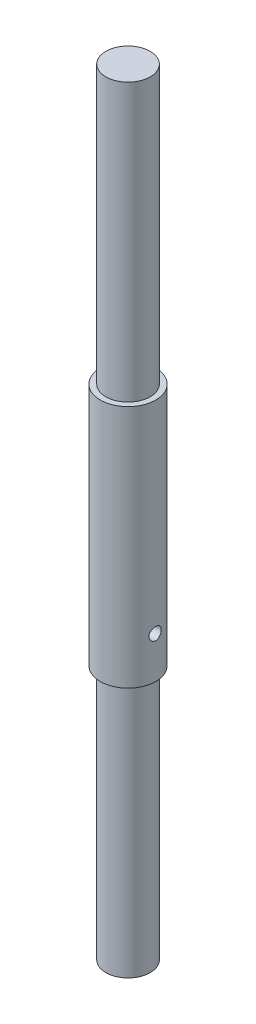
SolidWorks part; units mm, degrees
ref_plane "前视基准面" through (0, 0, 0) normal (0, 0, 1) x (1, 0, 0)
ref_plane "上视基准面" through (0, 0, 0) normal (0, 1, 0) x (1, 0, 0)
ref_plane "右视基准面" through (0, 0, 0) normal (1, 0, 0) x (0, 0, -1)
sketch "草图4" plane through (0, 0, 0) normal (0, 0, 1) x (1, 0, 0)
  line L0 (0, 0) -> (0, 8302.0677) construction
  line L1 (0, 125.0089) -> (4, 125.0089)
  line L2 (4, 125.0089) -> (4, 75.0089)
  line L3 (4, 75.0089) -> (5, 75.0089)
  line L4 (5, 75.0089) -> (5, 31.0089)
  line L5 (5, 31.0089) -> (4, 31.0089)
  line L6 (4, 31.0089) -> (4, -14.9911)
  line L7 (4, -14.9911) -> (0, -14.9911)
  line L8 (0, 125.0089) -> (0, -14.9911)
  dimension "D1" = 4
  dimension "D2" = 4
  dimension "D3" = 50
  dimension "D4" = 140
  dimension "D5" = 44
  dimension "D6" = 1
  dimension "D7" = 1
revolve "旋转1" add sketch "草图4" angle 360 about L0
sketch "草图5" plane through (0, 0, 0) normal (1, 0, 0) x (0, 0, -1)
  line L0 (-4, 31.0089) -> (4, 31.0089) construction
  circle A0 centre (0, 38.5089) radius 1.1
  dimension "D2" = 2.2
  dimension "D1" = 7.5
extrude "切除-拉伸1" cut sketch "草图5" against normal mid plane 20
